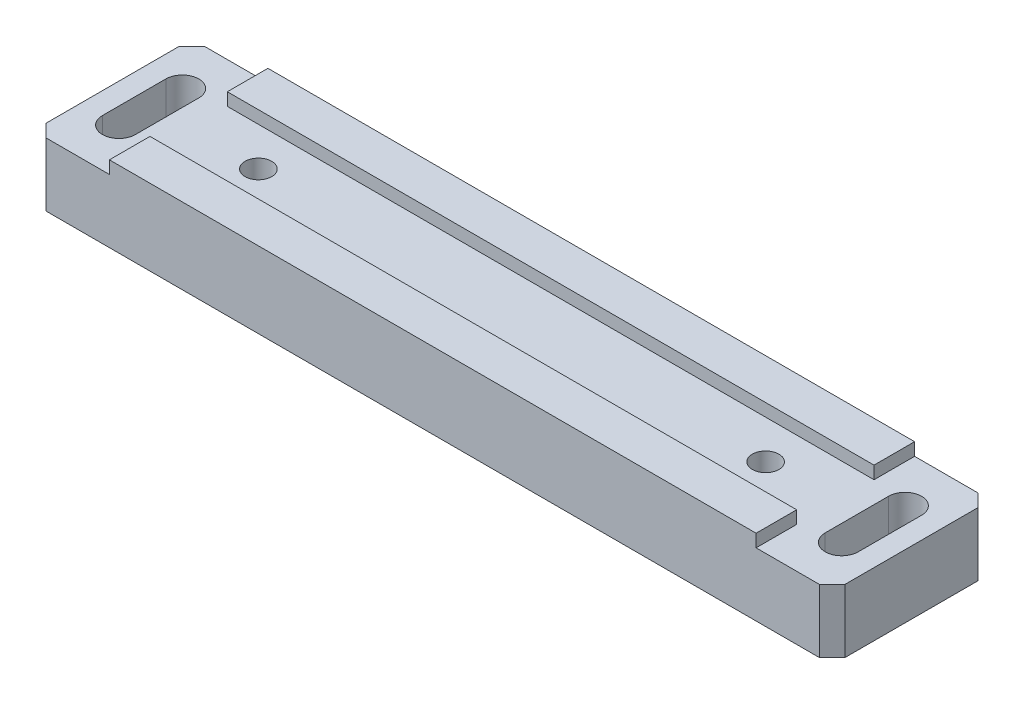
SolidWorks part; units mm, degrees
ref_plane "前视基准面" through (0, 0, 0) normal (0, 0, 1) x (1, 0, 0)
ref_plane "上视基准面" through (0, 0, 0) normal (0, 1, 0) x (1, 0, 0)
ref_plane "右视基准面" through (0, 0, 0) normal (1, 0, 0) x (0, 0, -1)
sketch "草图1" plane through (0, 0, 0) normal (0, 1, 0) x (1, 0, 0)
  line L1 (-63, 12.5) -> (63, 12.5)
  line L2 (-63, 12.5) -> (-63, -12.5)
  line L3 (-63, -12.5) -> (63, -12.5)
  line L4 (63, 12.5) -> (63, -12.5)
  line L5 (-63, 12.5) -> (63, -12.5) construction
  line L6 (-63, -12.5) -> (63, 12.5) construction
  point P0 (0, 0)
  dimension "D1" = 126
  dimension "D2" = 25
extrude "凸台-拉伸1" add sketch "草图1" along normal mid plane 12
sketch "草图2" plane through (0, 6, 0) normal (0, 1, 0) x (1, 0, 0)
  line L0 (-57, 5) -> (-57, -5) construction
  line L1 (-54.4, 5) -> (-54.4, -5)
  line L2 (-59.6, 5) -> (-59.6, -5)
  arc A0 (-54.4, 5) -> (-59.6, 5) centre (-57, 5) ccw
  arc A1 (-59.6, -5) -> (-54.4, -5) centre (-57, -5) ccw
  point P2 (-57, 0)
  dimension "D1" = 10
  dimension "D2" = 5.2
  dimension "D3" = 57
extrude "切除-拉伸1" cut sketch "草图2" against normal through all
mirror "镜向1" about plane through (0, 0, 0) normal (1, 0, 0) of "切除-拉伸1"
sketch "草图3" plane through (0, 6, 0) normal (0, 1, 0) x (1, 0, 0)
  line L1 (-80, 6.1) -> (80, 6.1)
  line L2 (-80, 6.1) -> (-80, -6.1)
  line L3 (-80, -6.1) -> (80, -6.1)
  line L4 (80, 6.1) -> (80, -6.1)
  line L5 (-80, 6.1) -> (80, -6.1) construction
  line L6 (-80, -6.1) -> (80, 6.1) construction
  point P0 (0, 0)
  dimension "D1" = 12.2
  dimension "D2" = 160
extrude "切除-拉伸2" cut sketch "草图3" against normal blind 2
chamfer "倒角1" distance 2 angle 45 4 edges at (-63, 0, -12.5) (63, 0, -12.5) (63, 0, 12.5) (-63, 0, 12.5)
hole_wizard "M5 螺纹孔1" positions "草图6" profile "草图5" tap size "M5" standard "GB" end condition through all
sketch "草图6" plane through (0, 4, 0) normal (0, 1, 0) x (1, 0, 0)
  point P0 (-40, 0)
  point P2 (40, 0)
  dimension "D1" = 80
  dimension "D2" = 40
sketch "草图5" plane through (-40, 4, 0) normal (1, 0, 0) x (0, 0, 1)
  line L0 (0, 0) -> (0, 10)
  line L1 (0, 10) -> (2.1, 10)
  line L2 (2.1, 10) -> (2.1, 0)
  line L5 (2.1, 0) -> (0, 0)
  line L11 (0, -6.35) -> (0, 107.95) construction
  dimension "通孔螺纹孔钻头直径" = 4.2
  dimension "通孔螺纹孔钻头深度" = 10
cosmetic thread "孔螺蚊线1" parameters "D2"=5
cosmetic thread "孔螺蚊线2" parameters "D2"=5
sketch "草图7" plane through (0, 6, 0) normal (0, 1, 0) x (1, 0, 0)
  line L0 (-57, 5) -> (-57, -5) construction
  line L1 (-52, 5) -> (-52, -5)
  line L2 (-62, 5) -> (-62, -5)
  line L3 (57, 5) -> (57, -5) construction
  line L4 (62, 5) -> (62, -5)
  line L5 (52, 5) -> (52, -5)
  arc A0 (-52, 5) -> (-62, 5) centre (-57, 5) ccw
  arc A1 (-62, -5) -> (-52, -5) centre (-57, -5) ccw
  arc A2 (62, 5) -> (52, 5) centre (57, 5) ccw
  arc A3 (52, -5) -> (62, -5) centre (57, -5) ccw
  point P4 (-57, 0)
  point P13 (57, 0)
  dimension "D1" = 5
  dimension "D2" = 5
extrude "切除-拉伸4" [suppressed] cut sketch "草图7" against normal blind 6
sketch "草图8" plane through (0, 6, 0) normal (0, 1, 0) x (1, 0, 0)
  line L0 (-63, 6.1) -> (-63, -6.1) construction
  line L1 (-93.8086, 47.2562) -> (-51, 47.2562)
  line L2 (-93.8086, 47.2562) -> (-93.8086, -18.9025)
  line L3 (-93.8086, -18.9025) -> (-51, -18.9025)
  line L4 (-51, 47.2562) -> (-51, -18.9025)
  line L5 (-93.8086, 47.2562) -> (-51, -18.9025) construction
  line L6 (-93.8086, -18.9025) -> (-51, 47.2562) construction
  line L7 (80.1877, 53.5107) -> (51, 53.5107)
  line L8 (80.1877, 53.5107) -> (80.1877, -17.0956)
  line L9 (80.1877, -17.0956) -> (51, -17.0956)
  line L10 (51, 53.5107) -> (51, -17.0956)
  line L11 (80.1877, 53.5107) -> (51, -17.0956) construction
  line L12 (80.1877, -17.0956) -> (51, 53.5107) construction
  line L13 (63, -6.1) -> (63, 6.1) construction
  point P0 (-72.4043, 14.1769)
  point P5 (65.5938, 18.2075)
  dimension "D1" = 12
  dimension "D2" = 12
extrude "切除-拉伸5" cut sketch "草图8" against normal blind 2
